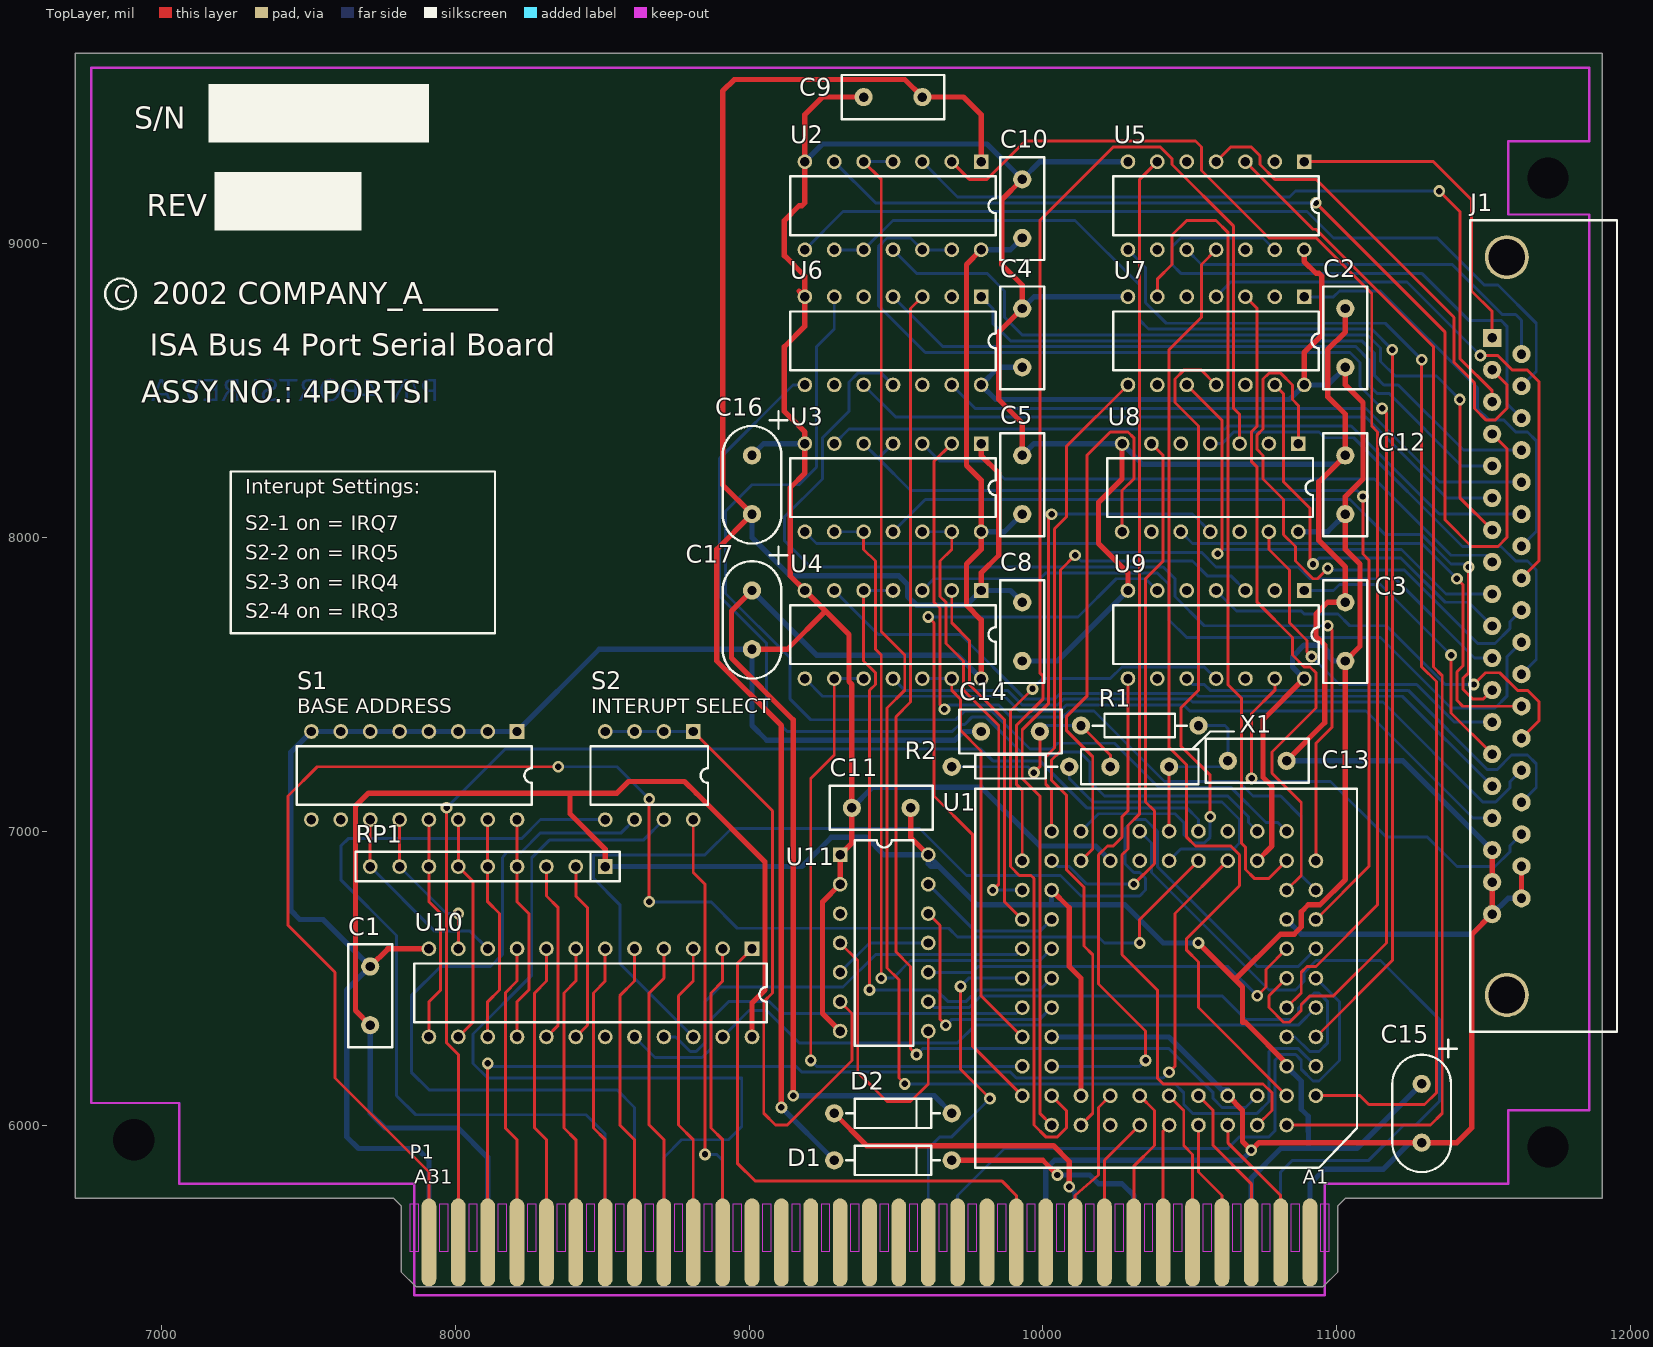
[diagram p0: TopLayer view]
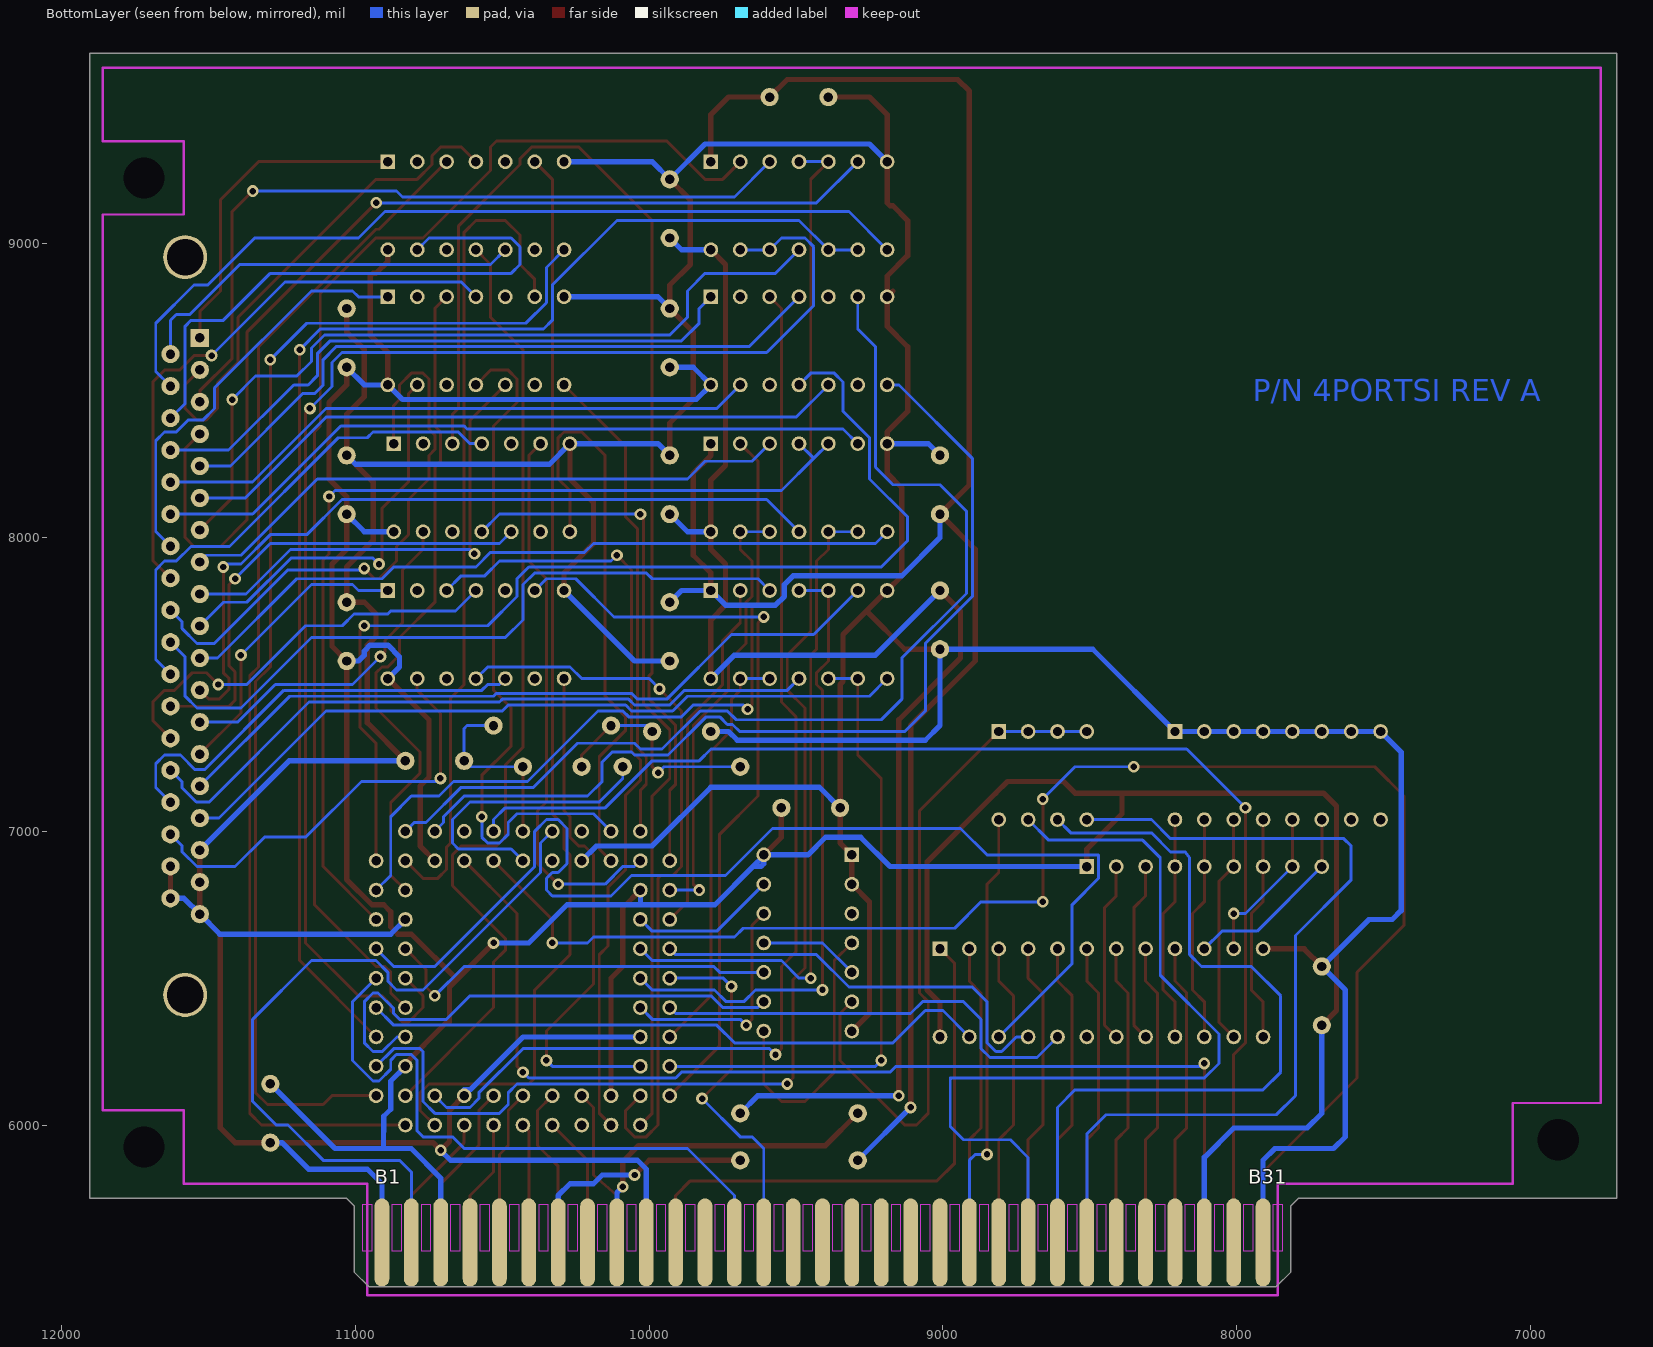
[diagram p1: BottomLayer view, seen from below]
# Altium PCB MISC95145.PcbDoc
Units mil, origin at the board's own origin, x right, y up, seen from the top; angles counter-clockwise.
Board outline 5200 x 4200 mil, 2 copper layers (TopLayer, BottomLayer); 36 components, 120 nets, 395 pads, 52 vias.

## Layer stack, top to bottom (the 12.6 mil dielectric is the usual default, probably not edited)
TopLayer: signal copper 1.4
Dielectric: core 12.6, FR-4, Dk 4.8
BottomLayer: signal copper 1.4

## Board outline
6705,9650 6705,5750 7790,5750 7815,5725 7815,5500 7865,5450 10955,5450 11005,5500 11005,5725 11030,5750 11905,5750 11905,9650

## Design rules (kind name [scope] priority, off if disabled: settings)
Clearance [All] p1: gap=10
ComponentClearance [All] p1 off: gap=10 collisioncheckmode=0
HoleSize [All] p1: absolutevalues=TRUE maxlimit=140 minlimit=1 maxpercent=80.000 minpercent=20.000
MinimumAnnularRing MinimumAnnularRing_Mtg [InPadClass('MTG')] p1: minimumring=-90
MinimumAnnularRing [All] p2: minimumring=9
PasteMaskExpansion PasteMaskExpansion_Edge [InComponent('P1')] p1: expansion=-150
PasteMaskExpansion [All] p2: expansion=0
PolygonConnect [All] p1: connectstyle=Relief reliefconductorwidth=10 reliefentries=4 polygonreliefangle="90 Angle"
RoutingLayers [All] p1: top layer=Vertical bottom layer=Horizontal
RoutingVias [All] p1: holewidth=22 width=40 viastyle="Through Hole" minholewidth=22 minwidth=40 maxholewidth=28 maxwidth=50
SolderMaskExpansion SolderMaskExpansion_Mtg [InPadClass('MTG')] p1: expansion=50
SolderMaskExpansion [All] p2: expansion=4
SupplyNets SupplyNets_1 [InNet('VCC')] p1: voltage=5.000
SupplyNets [InNet('GND')] p2: voltage=0.000
TestPointUsage [All] p1 off: valid=0 allowmultiple=FALSE
Testpoint [All] p1 off: side=15 testpointundercomponent=TRUE minsize=40 maxsize=100 preferedsize=60 minholesize=0 maxholesize=40 preferedholesize=32 testpointgrid=1 style=1023 order=1234567890
Width +12V [InNet('+12V')] p1: maxlimit=18 minlimit=18 preferedwidth=18
Width VCC [InNet('VCC')] p2: maxlimit=18 minlimit=18 preferedwidth=18
Width GND [InNet('GND')] p3: maxlimit=18 minlimit=18 preferedwidth=18
Width -12V [InNet('-12V')] p4: maxlimit=18 minlimit=18 preferedwidth=18
Width -12V_U/P [InNet('-12V_U/P')] p5: maxlimit=18 minlimit=18 preferedwidth=18
Width +12V_U/P [InNet('+12V_U/P')] p6: maxlimit=18 minlimit=18 preferedwidth=18
Width All [All] p7: maxlimit=10 minlimit=10 preferedwidth=10
14 further rules are at their usual default settings.

## Classes and differential pairs
pad class MTG: Free-1 Free-2 Free-3
net class A[0..2]: A0 A1 A2
net class D[0..7]: D0 D1 D2 D3 D4 D5 D6 D7

## Components (designator, comment, footprint, x,y, rotation, side; value= is the part's Value field where it differs from the comment)
C1 "0.1uF" RAD0.2 7710,6340 r90 top
C2 "0.1uF" RAD0.2 11030,8580 r90 top
C3 "0.1uF" RAD0.2 11030,7580 r90 top
C4 "0.1uF" RAD0.2 9930,8580 r90 top
C5 "0.1uF" RAD0.2 9930,8080 r90 top
C8 "0.1uF" RAD0.2 9930,7780 r270 top
C9 "0.1uF" RAD0.2 9590,9500 r180 top
C10 "0.1uF" RAD0.2 9930,9020 r90 top
C11 "0.1uF" RAD0.2 9550,7080 r180 top
C12 "0.1uF" RAD0.2 11030,8080 r90 top
C13 "20pF" RAD0.2 10630,7240 r0 top
C14 "50pF" RAD0.2 9990,7340 r180 top
C15 "10uF" "TANT 2M/2M" 11290,6140 r270 top
C16 "10uF" "TANT 2M/2M" 9010,8280 r270 top
C17 "10uF" "TANT 2M/2M" 9010,7820 r270 top
D1 "1N4004" DIODE0.4 9290,5880 r0 top
D2 "1N4004" DIODE0.4 9290,6040 r0 top
J1 "DB37" DB37RA/F 11530,8680 r270 top
P1 "CON AT62B" ECN-IBMXT 10910,5600 r0 top locked
R1 "1M" AXIAL0.4 10130,7360 r0 top
R2 "1K5" AXIAL0.4 10090,7220 r180 top
RP1 "10K" SIP9 8510,6880 r180 top
S1 "BASE ADDRESS" DIP16 8210,7340 r270 top
S2 "INTERUPT SELECT" DIP8 8810,7340 r270 top
U1 "TL16C554" PGA68X11_SKT 10430,6000 r270 top
U2 "1488" DIP14 9790,9280 r270 top
U3 "1488" DIP14 9790,8320 r270 top
U4 "1488" DIP14 9790,7820 r270 top
U5 "1489" DIP14 10890,9280 r270 top
U6 "1489" DIP14 9790,8820 r270 top
U7 "1489" DIP14 10890,8820 r270 top
U8 "1489" DIP14 10870,8320 r270 top
U9 "1489" DIP14 10890,7820 r270 top
U10 "P22V10" SDIP24 9010,6600 r270 top
U11 "74HC32" DIP14 9310,6920 r0 top
X1 "1.8432Mhz" XTAL1 10230,7220 r0 top

## Footprints (in the part's own frame and the unit in brackets; to place one, negate y for a bottom-side part, rotate by r counter-clockwise, add the part's x,y. Pads: shape width x height; smd on the part's side, far side on the other; paste and mask are expansions set on the pad)
AXIAL0.4 [mil]
  round 62 hole 32: 1(0,0) 2(400,0)
  silkscreen extent 40,-40 360,40
DB37RA/F [mil]
  round 150 hole 125: 0(-275,50) 0(2237,50)
  rect 62x62 hole 32: 1(0,0)
  round 62 hole 32: 2(109,0) 3(218,0) 4(327,0) 5(436,0) 6(545,0) 7(654,0) 8(763,0) 9(872,0) 10(981,0) 11(1090,0) 12(1199,0) 13(1308,0) 14(1417,0) 15(1526,0) 16(1635,0) 17(1744,0) 18(1853,0) 19(1962,0) 20(55,100) 21(164,100) 22(273,100) 23(382,100) 24(491,100) 25(600,100) 26(709,100) 27(818,100) 28(927,100) 29(1036,100) 30(1145,100) 31(1254,100) 32(1363,100) 33(1472,100) 34(1581,100) 35(1690,100) 36(1799,100) 37(1908,100)
  silkscreen extent -400,-75 2362,425
DIODE0.4 [mil]
  round 62 hole 32: A(0,0) K(400,0)
  silkscreen extent 40,-50 360,50
DIP8 [mil]
  rect 50x50 hole 32: 1(0,0)
  round 50 hole 32: 2(0,-100) 3(0,-200) 4(0,-300) 5(300,-300) 6(300,-200) 7(300,-100) 8(300,0)
  silkscreen extent 50,-350 250,50
DIP14 [mil]
  rect 50x50 hole 32: 1(0,0)
  round 50 hole 32: 2(0,-100) 3(0,-200) 4(0,-300) 5(0,-400) 6(0,-500) 7(0,-600) 8(300,-600) 9(300,-500) 10(300,-400) 11(300,-300) 12(300,-200) 13(300,-100) 14(300,0)
  silkscreen extent 50,-650 250,50
DIP16 [mil]
  rect 50x50 hole 32: 1(0,0)
  round 50 hole 32: 2(0,-100) 3(0,-200) 4(0,-300) 5(0,-400) 6(0,-500) 7(0,-600) 8(0,-700) 9(300,-700) 10(300,-600) 11(300,-500) 12(300,-400) 13(300,-300) 14(300,-200) 15(300,-100) 16(300,0)
  silkscreen extent 50,-750 250,50
ECN-IBMXT [mil]
  oval 50x300 smd: A1(0,0) A2(-100,0) A3(-200,0) A4(-300,0) A5(-400,0) A6(-500,0) A7(-600,0) A8(-700,0) A9(-800,0) A10(-900,0) A11(-1000,0) A12(-1100,0) A13(-1200,0) A14(-1300,0) A15(-1400,0) A16(-1500,0) A17(-1600,0) A18(-1700,0) A19(-1800,0) A20(-1900,0) A21(-2000,0) A22(-2100,0) A23(-2200,0) A24(-2300,0) A25(-2400,0) A26(-2500,0) A27(-2600,0) A28(-2700,0) A29(-2800,0) A30(-2900,0) A31(-3000,0)
  oval 50x300 smd far side: B1(0,0) B2(-100,0) B3(-200,0) B4(-300,0) B5(-400,0) B6(-500,0) B7(-600,0) B8(-700,0) B9(-800,0) B10(-900,0) B11(-1000,0) B12(-1100,0) B13(-1200,0) B14(-1300,0) B15(-1400,0) B16(-1500,0) B17(-1600,0) B18(-1700,0) B19(-1800,0) B20(-1900,0) B21(-2000,0) B22(-2100,0) B23(-2200,0) B24(-2300,0) B25(-2400,0) B26(-2500,0) B27(-2600,0) B28(-2700,0) B29(-2800,0) B30(-2900,0) B31(-3000,0)
PGA68X11_SKT [mil]
  round 50 hole 32: 1(0,0) 2(-100,0) 3(0,100) 4(-100,100) 5(0,200) 6(-100,200) 7(0,300) 8(-100,300) 9(0,400) 10(-100,500) 11(-100,400) 12(-200,500) 13(-200,400) 14(-300,500) 15(-300,400) 16(-400,500) 17(-400,400) 18(-500,500) 19(-500,400) 20(-600,500) 21(-600,400) 22(-700,500) 23(-700,400) 24(-800,500) 25(-800,400) 26(-900,500) 27(-1000,400) 28(-900,400) 29(-1000,300) 30(-900,300) 31(-1000,200) 32(-900,200) 33(-1000,100) 34(-900,100) 35(-1000,0) 36(-900,0) 37(-1000,-100) 38(-900,-100) 39(-1000,-200) 40(-900,-200) 41(-1000,-300) 42(-900,-300) 43(-1000,-400) 44(-900,-500) 45(-900,-400) 46(-800,-500) 47(-800,-400) 48(-700,-500) 49(-700,-400) 50(-600,-500) 51(-600,-400) 52(-500,-500) 53(-500,-400) 54(-400,-500) 55(-400,-400) 56(-300,-500) 57(-300,-400) 58(-200,-500) 59(-200,-400) 60(-100,-500) 61(0,-400) 62(-100,-400) 63(0,-300) 64(-100,-300) 65(0,-200) 66(-100,-200) 67(0,-100) 68(-100,-100)
  silkscreen extent -1145,-660 145,640
RAD0.2 [mil]
  round 62 hole 32: 1(0,0) 2(200,0)
  silkscreen extent -75,-75 275,75
SDIP24 [mil]
  rect 50x50 hole 32: 1(0,0)
  round 50 hole 32: 2(0,-100) 3(0,-200) 4(0,-300) 5(0,-400) 6(0,-500) 7(0,-600) 8(0,-700) 9(0,-800) 10(0,-900) 11(0,-1000) 12(0,-1100) 13(300,-1100) 14(300,-1000) 15(300,-900) 16(300,-800) 17(300,-700) 18(300,-600) 19(300,-500) 20(300,-400) 21(300,-300) 22(300,-200) 23(300,-100) 24(300,0)
  silkscreen extent 50,-1150 250,50
SIP9 [mil]
  rect 50x50 hole 32: 1(0,0)
  round 50 hole 32: 2(100,0) 3(200,0) 4(300,0) 5(400,0) 6(500,0) 7(600,0) 8(700,0) 9(800,0)
  silkscreen extent -50,-50 850,50
"TANT 2M/2M" [mil]
  round 62 hole 32: 1(0,0) 2(200,0)
  silkscreen extent -150,-100 300,120
XTAL1 [mil]
  round 62 hole 32: 1(0,0) 2(200,0)
  silkscreen extent -100,-60 300,60

## Free pads (board coordinates)
  round 50 hole 140: 1(6905,5950) 2(11720,5925) 3(11720,9225)

## Via types
v1: diameter 40, hole 22, TopLayer to BottomLayer, 52 vias

## Nets (pads, with @x,y where several pads share a name; then routed paths per layer and width w, separated by ;. In a path a pad name is that pad's centre, name@x,y a point inside that pad or via, vN(x,y) a via of type N, cw(c..) or ccw(c..) an arc to the next point about the centre after c; other vN are vias at no path point)
+12V: C5.1 C10.1 C17.1 D2.K U2.14 U3.14 U4.14 | length 5169.4
  TopLayer w18: C17.1 8940,7750 8940,7590 9150,7380 v1(9150,6100) ; U4.14 9790,7720 9740,7770 9740,7910 9790,7960 U3.14 9790,8196 9740,8246 9740,8930 U2.14
  BottomLayer w18: C17.1 9230,7600 9710,7600 U4.14 ; v1(9150,6100) 9630,6100 D2.K ; U3.14 9870,8020 C5.1 ; U2.14 9890,8980 C10.1
+12V_U/P: D2.A P1.B9 | length 1152.2
  TopLayer w18: D2.A 9400,5930 10036,5930 10090,5876 v1(10090,5790)
  BottomLayer w18: v1(10090,5790) 10100,5780 10110,5770 P1.B9
-12V: C8.1 C9.1 C16.2 D1.A U2.1 U3.1 U4.1 | length 6708.8
  TopLayer w18: v1(9110,6060) 9110,7360 8890,7580 8890,7960 C16.2 8910,8180 8910,9520 8950,9560 9530,9560 C9.1 9730,9500 9790,9440 U2.1 ; U4.1 9790,7880 9850,7940 9850,8220 9790,8280 U3.1
  BottomLayer w18: C16.2 9010,8000 9140,7870 9510,7870 9540,7840 9540,7800 9570,7770 9740,7770 U4.1 9890,7820 C8.1 ; v1(9110,6060) D1.A
-12V_U/P: D1.K P1.B7 | length 829.7
  TopLayer w18: D1.K 10000,5880 v1(10050,5830)
  BottomLayer w18: v1(10050,5830) 10160,5830 10190,5800 10270,5800 10310,5760 P1.B7
-CSA: U1.16 U10.23 | length 2152.5
  BottomLayer w10: U10.23 9000,6390 9060,6390 9170,6280 9710,6280 9770,6340 10870,6340 U1.16
-CSB: U1.20 U10.22 | length 3997.1
  BottomLayer w10: U10.22 8560,6550 8560,6750 8470,6840 8470,6920 8850,6920 8940,7010 9580,7010 9740,6850 10060,6850 10130,6780 10330,6780 10350,6800 10350,6840 10330,6860 10310,6860 10280,6890 10280,7010 10310,7040 10350,7040 10390,7000 10390,6880 10730,6540 10870,6540 U1.20
-CSC: U1.50 U10.21 | length 1467.7
  BottomLayer w10: U10.21 8750,6300 8800,6250 8820,6250 8850,6280 8850,6420 8900,6470 9320,6470 9430,6580 9910,6580 U1.50
-CSD: U1.54 U10.20 | length 1511.1
  BottomLayer w10: U10.20 8680,6230 8840,6230 8870,6260 8870,6360 8930,6420 9070,6420 9110,6380 9910,6380 U1.54
-RD: P1.B14 U1.52 | length 1245.4
  TopLayer w10: v1(9720,6472) 9720,6190 v1(9820,6090)
  BottomLayer w10: P1.B14 9610,5920 9650,5960 9690,5960 v1(9820,6090) ; v1(9720,6472) 9748,6500 U1.52
-WR: P1.B13 U1.18 | length 2197
  BottomLayer w10: P1.B13 9710,5760 9870,5920 10630,5920 10670,5960 10770,5960 10790,5980 10790,6220 10810,6240 10861,6240 10880,6221 10880,6190 10920,6150 10940,6150 11010,6220 11010,6420 U1.18
A0: P1.A31 U1.34 | length 5476.6
  TopLayer w10: P1.A31 7910,5840 7590,6160 7590,6520 7430,6680 7430,7120 7530,7220 v1(8350,7220) ; v1(8660,6760) v1(8660,7110) ; v1(10330,6620) 10330,6700 10370,6740 U1.34
  BottomLayer w10: v1(8350,7220) 8550,7220 v1(8660,7110) ; v1(8660,6760) 8870,6760 8960,6670 9680,6670 9710,6640 10190,6640 10210,6620 v1(10330,6620)
A1: P1.A30 U1.33 | length 4278.8
  TopLayer w10: v1(7970,7080) 7970,6280 8010,6240 P1.A30
  BottomLayer w10: v1(7970,7080) 8170,7280 9790,7280 9830,7240 9990,7240 10150,7080 10490,7080 10530,7040 U1.33
A2: P1.A29 U1.32 | length 3761.8
  TopLayer w10: P1.A29 v1(8110,6210) ; v1(10430,6180) 10450,6200 10450,6720 U1.32
  BottomLayer w10: v1(8110,6210) 8120,6200 9160,6200 9180,6180 9890,6180 9910,6160 10410,6160 v1(10430,6180)
CARD_ENABLE: U10.19
CTSA: U1.11 U5.11 | length 3331.4
  TopLayer w10: U5.11 10540,8930 10540,8750 10430,8640 10430,7286 10490,7226 10490,6980 10520,6950 10640,6950 10670,6920 10670,6815 10490,6635 10490,6595 10530,6555 10530,6400 U1.11
CTSB: U1.25 U7.3 | length 2272
  TopLayer w10: U7.3 10730,8780 10730,8380 10710,8360 10710,8260 10730,8240 10730,7780 10850,7660 10850,7600 10890,7560 10910,7560 10930,7540 10930,7420 10780,7270 10780,7198 10880,7098 10880,6850 U1.25
CTSC: U1.45 U8.6 | length 1896
  TopLayer w10: v1(10310,6820) 10380,6890 10380,7070 10350,7100 10350,7860 10410,7920 10410,8280 U8.6
  BottomLayer w10: U1.45 10050,6880 10090,6880 10150,6820 v1(10310,6820)
CTSD: U1.59 U9.8 | length 1747.7
  TopLayer w10: U9.8 10290,7070 10270,7050 10270,6980 10240,6950 10220,6950 10190,6920 10190,6480 10350,6320 v1(10350,6220)
  BottomLayer w10: U1.59 10330,6200 v1(10350,6220)
D0: P1.A9 U1.66 | length 552.9
  TopLayer w10: P1.A9 10110,5760 10190,5830 10190,6060 U1.66
D1: P1.A8 U1.67 | length 449.7
  TopLayer w10: P1.A8 10210,5880 U1.67
D2: P1.A7 U1.68 | length 549.7
  TopLayer w10: P1.A7 10310,5860 10380,5930 10380,6050 U1.68
D3: P1.A6 U1.1 | length 408.3
  TopLayer w10: P1.A6 10410,5980 U1.1
D4: P1.A5 U1.2 | length 533.1
  TopLayer w10: U1.2 10480,6050 10480,5930 10510,5900 P1.A5
D5: P1.A4 U1.3 | length 433.1
  TopLayer w10: U1.3 10530,5840 10610,5760 P1.A4
D6: P1.A3 U1.4 | length 574.6
  TopLayer w10: U1.4 10580,6050 10580,5930 10710,5800 P1.A3
D7: P1.A2 U1.5 | length 474.6
  TopLayer w10: U1.5 10630,5940 10810,5760 P1.A2
DCDA: U1.9 U5.3 | length 4069.9
  TopLayer w10: U5.3 10920,9050 10930,9050 11330,8650 11330,7560 11360,7530 11360,6040 11320,6000 U1.9
DCDB: U1.27 U6.6 | length 3625.9
  BottomLayer w10: U6.6 9290,8710 9230,8650 9230,8240 9170,8180 9010,8180 8920,8090 8920,7810 9140,7590 9140,7450 9210,7380 9704,7380 9734,7410 9826,7410 9956,7280 10030,7280 10050,7300 10244,7300 10394,7150 10640,7150 10760,7030 10800,7030 U1.27
DCDC: U1.43 U7.8 | length 1644.3
  TopLayer w10: U1.43 10030,7140 10010,7160 10010,7254 10040,7284 10040,8030 10080,8070 10080,8310 U7.8
DCDD: U1.61 U8.11 | length 2727.7
  TopLayer w10: U1.61 9990,6040 9990,7120 9930,7180 9930,7346 10020,7436 10020,8070 v1(10030,8080)
  BottomLayer w10: v1(10030,8080) 10510,8080 U8.11
DSRA: U1.10 U5.8 | length 4180.9
  TopLayer w10: U1.10 11080,6100 11110,6070 11300,6070 11340,6110 11340,7510 11290,7560 v1(11290,8606)
  BottomLayer w10: U5.8 10350,8920 10350,8800 10420,8730 11166,8730 v1(11290,8606)
DSRB: U1.26 U6.11 | length 3643.6
  TopLayer w10: U1.26 10930,7300 10984,7354 10984,7686 v1(10970,7700)
  BottomLayer w10: U6.11 9450,8560 9370,8560 9340,8530 9340,8430 9250,8340 9250,8200 9120,8070 9120,7990 9210,7900 10410,7900 10450,7860 10450,7800 10550,7700 v1(10970,7700)
DSRC: U1.44 U8.3 | length 3865.1
  TopLayer w10: U1.44 9930,7140 9910,7160 9910,7360 10000,7450 10000,7530 9990,7540 9990,9080 10240,9330 10400,9330 10440,9290 10440,9270 10650,9060 10650,8440 10670,8420 U8.3
DSRD: U1.60 U9.6 | length 2613
  TopLayer w10: v1(9610,7730) 9630,7710 9630,7120 9760,6990 9760,6270 U1.60
  BottomLayer w10: v1(9610,7730) 10120,7730 10250,7860 10350,7860 U9.6
DTRA: U1.12 U2.4 U2.5 | length 5028.1
  TopLayer w10: U2.5 9450,9220 9450,7680 9530,7600 9530,7480 9470,7420 9470,6535 9510,6495 9510,6160 v1(9530,6140)
  BottomLayer w10: U2.5 U2.4 ; v1(9530,6140) 10450,6140 10480,6110 10480,6070 10510,6040 10730,6040 10770,6080 10770,6250 10780,6260 10870,6260 U1.12
DTRB: U1.24 U3.2 | length 2608.8
  TopLayer w10: v1(9665,7416) 9650,7431 9650,7760 9630,7780 9630,8260 U3.2
  BottomLayer w10: v1(9665,7416) 9679,7430 9850,7430 9890,7390 10070,7390 10090,7410 10174,7410 10414,7170 10666,7170 10716,7120 10810,7120 10880,7050 10880,6850 U1.24
DTRC: U1.46 U3.12 U3.13 | length 1527.7
  TopLayer w10: U3.13 9690,7960 9650,7920 9650,7800 9670,7780 9670,7640 9730,7580 9730,7480 9850,7360 9850,6820 v1(9830,6800)
  BottomLayer w10: U3.12 U3.13 ; v1(9830,6800) U1.46
DTRD: U1.58 U4.9 U4.10 | length 2161.4
  TopLayer w10: v1(9210,6220) 9210,7180 9290,7260 U4.9
  BottomLayer w10: v1(9210,6220) 9230,6200 U1.58 ; U4.9 U4.10
GND: C1.2 C2.2 C3.2 C4.2 C5.2 C8.2 C9.2 C10.2 C11.2 C12.2 C13.2 C14.2 C15.2 C16.1 C17.2 J1.17 J1.18 J1.19 J1.36 J1.37 P1.B1 P1.B10 P1.B31 S1.1 S1.2 S1.3 S1.4 S1.5 S1.6 S1.7 S1.8 U1.6 U1.23 U1.40 U1.57 U2.7 U3.7 U4.7 U5.7 U6.7 U7.7 U8.7 U9.7 U10.12 U11.1 U11.2 U11.7 | length 23020
  TopLayer w18: C1.2 7770,6600 U10.12 ; C17.2 9130,7620 9260,7750 ; 9170,8840 U6.7 ; U11.7 9250,6380 9250,6760 U11.2 U11.1 9350,6960 C11.2 9350,7500 9340,7510 9340,7670 9260,7750 ; C9.2 9250,9500 9190,9440 U2.7 9190,9140 9180,9130 9170,9130 9120,9080 9120,8960 9190,8890 U6.7 ; C5.2 9930,8390 9850,8470 9850,8700 C4.2 9930,8860 9860,8930 9860,9150 C10.2 ; U8.7 10270,8200 10190,8120 10190,7980 10290,7880 U9.7 ; U1.6 10680,6050 10680,5944 v1(10710,5914) 10736,5940 C15.2 11410,5940 11460,5990 11460,6648 J1.19 J1.18 J1.17 ; C13.2 10960,7370 10960,7634 10930,7664 10930,7740 10970,7780 C3.2 11030,7900 10940,7990 10940,8190 C12.2 11030,8420 10970,8480 10970,8640 11030,8700 C2.2 ; J1.37 J1.36 ; U6.7 9190,8720 9120,8650 9120,8430 9190,8360 U3.7 9190,8220 9140,8170 9140,7870 U4.7 9260,7750
  BottomLayer w18: P1.B31 7910,5880 7870,5920 7670,5920 7630,5960 7630,6460 C1.2 7550,6700 7470,6700 7440,6730 7440,7270 S1.8 S1.7 S1.6 S1.5 S1.4 S1.3 S1.2 S1.1 8490,7620 C17.2 9010,7360 9060,7310 9700,7310 9730,7340 C14.2 ; C16.1 9050,8320 U3.7 ; U2.7 9250,9340 9810,9340 C10.2 9990,9280 U5.7 ; C11.2 9420,7150 9790,7150 9990,6950 10180,6950 U1.40 ; C8.2 10050,7580 U9.7 ; C5.2 9970,8320 U8.7 10340,8250 11000,8250 C12.2 ; C4.2 9970,8820 U7.7 ; P1.B10 10010,5850 10040,5880 10676,5880 v1(10710,5914) ; U1.57 10430,6300 10610,6120 10630,6120 U1.6 ; U1.23 10880,6650 11462,6650 J1.19 11584,6772 J1.37 ; C13.2 11226,7240 J1.17 ; P1.B1 10910,5800 10960,5850 11160,5850 11250,5940 C15.2
INTA: U1.15 U11.9 | length 1790.8
  BottomLayer w10: U11.9 9630,6400 9750,6400 9790,6440 10610,6440 10690,6360 10850,6360 10870,6380 10870,6397 10923,6450 10940,6450 10970,6420 10970,6280 10940,6250 10909,6250 10859,6300 U1.15
INTB: U1.21 U11.10 | length 1371.1
  TopLayer w10: v1(10730,6440) 10760,6470 10760,6530 U1.21
  BottomLayer w10: U11.10 9760,6520 9780,6540 10630,6540 v1(10730,6440)
INTC: U1.49 U11.13 | length 502.8
  BottomLayer w10: U11.13 9770,6660 9990,6660 U1.49
INTD: U1.55 U11.12 | length 789.7
  TopLayer w10: U11.12 9650,6680 9650,6360 v1(9670,6340)
  BottomLayer w10: v1(9670,6340) 9690,6360 9990,6360 U1.55
J1: J1.1 U5.1 | length 1122.8
  TopLayer w10: U5.1 11330,9280 11460,9150 11460,8840 11530,8770 J1.1
J2: J1.20 U5.10 | length 1354.4
  BottomLayer w10: U5.10 10540,8930 11394,8930 11564,8760 11610,8760 11630,8740 J1.20
J3: J1.2 U5.4 | length 1722.4
  TopLayer w10: U5.4 10640,9330 10710,9330 10740,9300 10740,9270 10790,9220 10930,9220 11400,8750 11400,8597 11470,8527 11470,8440 11510,8400 11540,8400 11580,8440 11580,8521 J1.2
J4: J1.21 U2.8 | length 2936
  BottomLayer w10: U2.8 9320,9110 10900,9110 10990,9020 11343,9020 11503,8860 11550,8860 11680,8730 11680,8566 J1.21
J5: J1.3 U2.3 | length 2610.5
  TopLayer w10: v1(11350,9180) 11420,9110 11420,8610 11530,8500 J1.3
  BottomLayer w10: U2.3 9710,9160 10840,9160 10860,9180 v1(11350,9180)
J6: J1.22 U5.13 | length 1999.7
  BottomLayer w10: U5.13 10750,9020 10470,9020 10440,8990 10440,8930 10470,8900 11290,8900 11450,8740 11560,8740 11580,8720 11580,8457 J1.22
J7: J1.4 U2.6 | length 3593.1
  TopLayer w10: v1(10929,9140) 11370,8699 11370,8060 11460,7970 11550,7970 11580,8000 11580,8303 J1.4
  BottomLayer w10: U2.6 9430,9140 v1(10929,9140)
J8: J1.23 U6.1 | length 2129.4
  BottomLayer w10: U6.1 9830,8780 9830,8730 9890,8670 11086,8670 11130,8626 11130,8551 11161,8520 11210,8520 11432,8298 J1.23
J11: J1.5 U6.4 | length 2329
  BottomLayer w10: U6.4 9660,8650 11066,8650 11110,8606 11110,8520 11140,8490 11180,8490 11426,8244 J1.5
J12: J1.24 U6.13 | length 2077.1
  BottomLayer w10: U6.13 9770,8440 11100,8440 11351,8189 J1.24
J13: J1.6 U6.10 | length 2299.5
  BottomLayer w10: U6.10 9500,8410 11100,8410 11375,8135 J1.6
J14: J1.25 U3.6 | length 2489.1
  BottomLayer w10: U3.6 9340,8370 10620,8370 10630,8380 11050,8380 11350,8080 J1.25
J15: J1.7 U2.11 | length 2710.5
  TopLayer w10: v1(11420,8470) 11420,8136 J1.7
  BottomLayer w10: U2.11 9570,8900 9810,8900 9870,8840 9870,8750 9930,8690 11106,8690 11150,8646 11150,8600 11200,8550 11340,8550 v1(11420,8470)
J16: J1.26 U7.1 | length 1430.2
  BottomLayer w10: U7.1 10990,8820 11010,8840 11150,8840 11480,8510 11480,8440 11520,8400 11570,8400 11610,8360 11650,8360 11680,8330 11680,8021 J1.26
J17: J1.8 U3.3 | length 2106.9
  BottomLayer w10: U3.3 9650,8260 9810,8260 9870,8200 11130,8200 11390,7940 11507,7940 J1.8
J18: J1.27 U7.4 | length 1954.4
  TopLayer w10: v1(11490,8620) 11549,8620 11599,8570 11650,8570 11690,8530 11690,7922 J1.27
  BottomLayer w10: U7.4 10640,8870 11240,8870 v1(11490,8620)
J21: J1.9 U7.10 | length 1635.1
  TopLayer w10: U7.10 10610,8400 10610,7960 v1(10595,7945)
  BottomLayer w10: v1(10595,7945) 10610,7960 11221,7960 11373,7808 J1.9
J22: J1.28 U8.1 | length 1990.5
  TopLayer w10: U8.1 10870,8450 10850,8470 10850,8520 10810,8560 10770,8560 10750,8540 10750,8370 10730,8350 10730,8300 10750,8280 10750,8200 10820,8130 10820,8010 10860,7970 10860,7920 10920,7860 10935,7860 v1(10970,7895)
  BottomLayer w10: v1(10970,7895) 10975,7890 11231,7890 11481,7640 11540,7640 11590,7690 11590,7713 J1.28
J23: J1.10 U7.13 | length 1377.8
  TopLayer w10: U7.13 10820,8490 10820,8190 10910,8100 10910,7920 v1(10920,7910)
  BottomLayer w10: v1(10920,7910) 10940,7930 11220,7930 11370,7780 11449,7780 J1.10
J24: J1.29 U4.3 | length 2497
  BottomLayer w10: U4.3 9630,7860 9990,7860 10010,7880 10390,7880 10430,7840 10430,7720 10490,7660 11150,7660 11390,7420 11540,7420 11580,7460 11580,7594 J1.29
J25: J1.11 U3.8 | length 2518.1
  BottomLayer w10: U3.8 9230,7980 10190,7980 10220,7950 10540,7950 10590,7900 10870,7900 10910,7860 11200,7860 11470,7590 J1.11
J26: J1.30 U8.4 | length 1697
  BottomLayer w10: U8.4 10610,8320 10650,8360 10940,8360 10960,8340 11059,8340 11429,7970 11560,7970 11610,7920 11650,7920 11680,7890 11680,7585 J1.30
J27: J1.12 U3.11 | length 2651.5
  TopLayer w10: v1(11450,7900) 11450,7540 11430,7520 11430,7485 11465,7450 11499,7450 J1.12
  BottomLayer w10: U3.11 9600,8130 11046,8130 11166,8010 11290,8010 11390,7910 11440,7910 v1(11450,7900)
J28: J1.31 U8.10 | length 1665.1
  TopLayer w10: v1(11410,7860) 11430,7840 11430,7563 11410,7543 11410,7446 11430,7426 J1.31
  BottomLayer w10: U8.10 10510,7980 11290,7980 v1(11410,7860)
J31: J1.13 U8.13 | length 1192.4
  TopLayer w10: U8.13 10770,7960 10840,7890 10840,7710 10900,7650 10900,7610 v1(10915,7595)
  BottomLayer w10: v1(10915,7595) 11010,7500 11273,7500 11401,7372 J1.13
J32: J1.32 U9.4 | length 1438.4
  TopLayer w10: v1(11467,7500) 11507,7540 11556,7540 11616,7480 11650,7480 11690,7440 11690,7377 J1.32
  BottomLayer w10: U9.4 10660,7750 10880,7750 10890,7740 11005,7740 11045,7700 11170,7700 11370,7500 v1(11467,7500)
J33: J1.14 U9.1 | length 1002.7
  TopLayer w10: v1(11390,7600) 11390,7403 J1.14
  BottomLayer w10: U9.1 10990,7820 11010,7840 11150,7840 v1(11390,7600)
J34: J1.33 U4.11 | length 2387
  BottomLayer w10: U4.11 9530,7480 9880,7480 9930,7430 10050,7430 10070,7450 10500,7450 10510,7440 11158,7440 11498,7100 11542,7100 11590,7148 11590,7168 J1.33
J35: J1.15 U4.6 | length 2532.4
  BottomLayer w10: U4.6 9440,7670 9720,7670 9940,7450 10040,7450 10060,7470 10520,7470 10530,7460 11224,7460 J1.15
J36: J1.34 U9.10 | length 1503.3
  BottomLayer w10: U9.10 10510,7500 10550,7500 10570,7480 11244,7480 11514,7210 11546,7210 11596,7260 11650,7260 11680,7230 11680,7149 J1.34
J37: J1.16 U4.8 | length 2553.3
  BottomLayer w10: U4.8 9250,7460 9870,7460 9920,7410 10060,7410 10080,7430 10480,7430 10500,7410 11100,7410 11465,7045 J1.16
J38: J1.35 U9.13 | length 1473.3
  TopLayer w10: v1(10711,7180) 10711,7401 10790,7480 U9.13
  BottomLayer w10: v1(10711,7180) 10721,7170 10980,7170 11170,6980 11310,6980 11410,6880 11540,6880 11590,6930 11590,6950 J1.35
NetC13_1: C13.1 R1.2 U1.35 X1.2 | length 642.4
  TopLayer w10: U1.35 X1.2
  BottomLayer w10: X1.2 10610,7220 C13.1 10630,7350 10620,7360 R1.2
NetC14_1: C14.1 R1.1 R2.2 X1.1 | length 766.3
  TopLayer w10: v1(9970,7200) 9990,7220 C14.1 ; R1.1 10230,7260 X1.1
  BottomLayer w10: R2.2 9950,7220 v1(9970,7200) ; C14.1 10010,7360 R1.1
NetP1_A11: P1.A11 U10.1 | length 1906.3
  TopLayer w10: U10.1 8960,6550 8960,5870 9020,5810 9860,5810 9910,5760 P1.A11
NetP1_A21: P1.A21 U10.2 | length 1033.1
  TopLayer w10: P1.A21 8910,5950 8870,5990 8870,6450 8910,6490 U10.2
NetP1_A22: P1.A22 U10.3 | length 1041.4
  TopLayer w10: P1.A22 8810,5950 8760,6000 8760,6440 8810,6490 U10.3
NetP1_A23: P1.A23 U10.4 | length 1041.4
  TopLayer w10: P1.A23 8710,5950 8660,6000 8660,6450 8710,6500 U10.4
NetP1_A24: P1.A24 U10.5 | length 1041.4
  TopLayer w10: P1.A24 8610,5950 8560,6000 8560,6440 8610,6490 U10.5
NetP1_A25: P1.A25 U10.6 | length 1033.1
  TopLayer w10: P1.A25 8510,5950 8470,5990 8470,6450 8510,6490 U10.6
NetP1_A26: P1.A26 U10.7 | length 1033.1
  TopLayer w10: P1.A26 8410,5950 8370,5990 8370,6450 8410,6490 U10.7
NetP1_A27: P1.A27 U10.8 | length 1033.1
  TopLayer w10: P1.A27 8310,5950 8270,5990 8270,6450 8310,6490 U10.8
NetP1_A28: P1.A28 U10.9 | length 1033.1
  TopLayer w10: P1.A28 8210,5950 8170,5990 8170,6450 8210,6490 U10.9
NetP1_B21: P1.B21 S2.8 | length 1504.9
  TopLayer w10: S2.8 8810,6860 8850,6820 v1(8850,5900)
  BottomLayer w10: v1(8850,5900) 8890,5900 8910,5880 P1.B21
NetP1_B23: P1.B23 S2.7 | length 2993
  BottomLayer w10: P1.B23 8710,5890 8770,5950 8930,5950 8975,5995 8975,6155 ; S2.7 8640,6970 8320,6970 8260,6910 8260,6510 8060,6310 8060,6210 8110,6160 8970,6160 ; 8970,6160 8975,6155 ; 8970,6160 8975,6160 8975,6155
NetP1_B24: P1.B24 S2.6 | length 2733.3
  BottomLayer w10: P1.B24 8610,6060 8550,6120 7910,6120 7850,6180 7850,6440 7950,6540 8120,6540 8160,6580 8160,6910 8175,6930 8225,6930 8290,6995 8565,6995 S2.6
NetP1_B25: P1.B25 S2.5 | length 3014.8
  BottomLayer w10: P1.B25@8510,5585 8510,5970 8445,6035 7865,6035 7800,6100 7800,6645 7610,6835 7610,6950 7635,6975 8225,6975 8290,7040 S2.5
NetR2_1: R2.1 U1.36 | length 1022.8
  BottomLayer w10: R2.1 10090,7180 10170,7100 10610,7100 10670,7040 10670,6960 10650,6940 10470,6940 U1.36
NetRP1_2: RP1.2 U10.18 | length 613.1
  TopLayer w10: U10.18 8450,6340 8450,6740 8410,6780 RP1.2
NetRP1_3: RP1.3 U10.17 | length 613.1
  TopLayer w10: U10.17 8350,6340 8350,6740 8310,6780 RP1.3
NetRP1_4: RP1.4 S1.16 U10.16 | length 773.1
  TopLayer w10: U10.16 8210,6420 8250,6460 8250,6720 8210,6760 RP1.4 S1.16
NetRP1_5: RP1.5 S1.15 U10.15 | length 773.1
  TopLayer w10: U10.15 8110,6420 8150,6460 8150,6720 8110,6760 RP1.5 S1.15
NetRP1_6: RP1.6 S1.14 U10.14 | length 781.4
  TopLayer w10: U10.14 8060,6350 8060,6830 RP1.6 S1.14
NetRP1_7: RP1.7 S1.13 U10.13 | length 773.1
  TopLayer w10: U10.13 7910,6420 7950,6460 7950,6720 7910,6760 RP1.7 S1.13
NetRP1_8: RP1.8 S1.12 U10.11 | length 546.3
  TopLayer w10: RP1.8 S1.12 ; U10.11 v1(8010,6720)
  BottomLayer w10: RP1.8 7970,6720 v1(8010,6720)
NetRP1_9: RP1.9 S1.11 U10.10 | length 676
  TopLayer w10: RP1.9 S1.11
  BottomLayer w10: RP1.9 7930,6660 8050,6660 U10.10
NetS2_1: S2.1 S2.2 S2.3 S2.4 U11.6 | length 2348.5
  TopLayer w10: S2.1 9080,7070 9080,6450 9050,6420 9050,6040 9090,6000 9130,6000 9350,6220 9350,6380 U11.6
  BottomLayer w10: S2.4 S2.3 S2.2 S2.1
NetU11_4: U11.4 U11.8 | length 951.1
  TopLayer w10: U11.4 9370,6560 9370,6180 9470,6080 9550,6080 9610,6140 U11.8
NetU11_5: U11.5 U11.11 | length 341.4
  BottomLayer w10: U11.5 9410,6620 U11.11
RESET: P1.B2 U1.37 | length 2603.5
  BottomLayer w10: U1.37 10370,6960 10370,6860 10770,6460 10860,6460 10890,6490 10890,6520 10930,6560 11150,6560 11350,6360 11350,6080 11270,6000 11230,6000 11110,5880 10850,5880 10810,5840 P1.B2
RIA: U1.8 U6.3 | length 3925.7
  TopLayer w10: v1(9570,6240) 9550,6260 9550,6540 9500,6590 9500,7390 9550,7440 9550,8780 U6.3
  BottomLayer w10: v1(9570,6240) 9590,6260 10430,6260 10580,6110 10580,6090 10610,6060 10690,6060 U1.8
RIB: U1.28 U7.6 | length 2830.1
  TopLayer w10: U7.6 10390,8880 10440,8930 10440,9030 10490,9080 10590,9080 10630,9040 10630,7500 10676,7454 10676,6960 10690,6946 10690,6870 10720,6840 10770,6840 U1.28
RIC: U1.42 U8.8 | length 2000.8
  TopLayer w10: U1.42 10170,6940 10170,7254 10080,7344 10080,7390 10150,7460 10150,8280 10230,8360 10290,8360 10310,8340 10310,8200 10270,8160 U8.8
RID: U1.62 U9.11 | length 2515
  TopLayer w10: v1(9965,7485) 9890,7410 9890,6880 9920,6850 9960,6850 9970,6840 9970,6000 10010,5960 10050,5960 10080,5990 10080,6050 U1.62
  BottomLayer w10: v1(9965,7485) 10000,7520 10230,7520 10270,7560 10550,7560 U9.11
RTSA: U1.14 U2.9 U2.10 | length 4641.7
  TopLayer w10: U1.14 11190,6560 v1(11190,8640)
  BottomLayer w10: U2.9 U2.10 9490,9080 10110,9080 10330,8860 10330,8740 10360,8710 11120,8710 v1(11190,8640)
RTSB: U1.22 U3.4 U3.5 | length 3438.8
  TopLayer w10: U1.22 11110,6880 11110,7924 11090,7944 v1(11090,8140)
  BottomLayer w10: U3.4 9440,8270 ; v1(11090,8140) 11070,8160 9550,8160 9440,8270 ; 9440,8270 U3.5 9440,8270
RTSC: U1.48 U4.2 | length 1219.4
  TopLayer w10: U4.2 9690,7710 9750,7650 9750,7500 9870,7380 9870,6760 U1.48
RTSD: U1.56 U4.12 U4.13 | length 1419.4
  TopLayer w10: U4.13 9690,7480 9720,7450 9720,7344 9790,7274 9790,6440 U1.56
  BottomLayer w10: U4.12 U4.13
RXA: U1.7 U5.6 | length 3760.8
  TopLayer w10: U5.6 10330,9220 10330,7060 10290,7020 10290,6940 10270,6920 10270,6580 10390,6460 10390,6160 10410,6140 10750,6140 10780,6110 10780,6050 U1.7
RXB: U1.29 U6.8 | length 3259.7
  BottomLayer w10: U6.8 9150,8520 8900,8270 8900,7800 9060,7640 9060,7410 9130,7340 9692,7340 9716,7364 9734,7364 9760,7390 9806,7390 9936,7260 10050,7260 10060,7270 10126,7270 10160,7236 10160,7170 10210,7120 10630,7120 10700,7050 10700,7030 U1.29
RXC: U1.41 U7.11 | length 2370.5
  TopLayer w10: v1(10570,7050) 10570,7191 10470,7291 10470,7420 10530,7480 10530,8380 10450,8460 10450,8540 10480,8570 10540,8570 U7.11
  BottomLayer w10: U1.41 10190,7060 10450,7060 10480,7030 10480,6990 10510,6960 10550,6960 10570,6980 v1(10570,7050)
RXD: U1.63 U9.3 | length 2677.4
  TopLayer w10: v1(10110,7940) 10060,7890 10060,7273 10030,7243 10030,7174 10080,7124 10080,6870 10140,6810 10140,6610 10170,6580 10170,6040 U1.63
  BottomLayer w10: v1(10110,7940) 10130,7920 10510,7920 10560,7870 10640,7870 U9.3
TXA: U1.17 U2.2 | length 4355.8
  TopLayer w10: U2.2 9750,9220 9810,9220 9940,9350 10520,9350 10540,9330 10540,9250 10770,9020 10931,9020 11120,8831 11120,8380 11140,8360 11140,6750 10930,6540 10900,6540 10880,6520 10880,6450 U1.17
TXB: U1.19 U2.12 U2.13 | length 4881.7
  TopLayer w10: U1.19 10770,6440 10770,6400 10820,6350 10840,6350 10880,6390 10880,6410 10910,6440 10990,6440 11170,6620 11170,8425 v1(11155,8440)
  BottomLayer w10: U2.13 U2.12 9550,9020 9470,9020 9440,8990 9440,8790 9600,8630 11046,8630 11080,8596 11080,8515 v1(11155,8440)
TXC: U1.51 U3.9 U3.10 | length 2266.3
  TopLayer w10: U3.10 9390,7960 9430,7920 9430,7620 9450,7600 v1(9450,6500)
  BottomLayer w10: U3.9 U3.10 ; v1(9450,6500) 9490,6500 9550,6560 9990,6560 U1.51
TXD: U1.53 U4.4 U4.5 | length 2154.6
  TopLayer w10: U4.5 9390,7580 9430,7540 9430,7500 9410,7480 v1(9410,6460)
  BottomLayer w10: U4.5 U4.4 ; v1(9410,6460) 9638,6460 9678,6420 9738,6420 9778,6460 9990,6460 U1.53
VCC: C1.1 C2.1 C3.1 C4.1 C11.1 C12.1 C15.1 P1.B3 P1.B29 RP1.1 U1.13 U1.30 U1.47 U1.64 U5.14 U6.14 U7.14 U8.14 U9.14 U10.24 U11.14 | length 14961.1
  TopLayer w18: C1.1 7660,6390 7660,7086 7704,7130 8390,7130 ; RP1.1 8510,6940 8390,7060 8390,7130 ; U10.24 9010,6416 9054,6460 9054,6896 8820,7130 8780,7170 8590,7170 8550,7130 8390,7130 ; C11.1 9550,6980 U11.14 ; U1.47 10090,6740 10090,6540 10130,6500 U1.64 ; v1(10530,6620) 10655,6495 ; U1.30 10780,6950 10780,7154 10750,7184 10750,7380 U9.14 ; U1.13 10840,6200 10690,6350 10680,6350 10680,6470 ; U7.14 10890,8630 10950,8690 10950,8890 10940,8900 10930,8900 10890,8940 U5.14 ; C2.1 11030,8520 11090,8460 11090,8200 11030,8140 C12.1 11030,7960 11080,7910 11080,7630 C3.1 11030,6836 10944,6750 10904,6750 10880,6726 10880,6674 10856,6650 10810,6650 10655,6495 ; 10655,6495 10680,6470 ; 10655,6495 10680,6470
  BottomLayer w18: C1.1 7710,6040 7760,5990 8010,5990 8110,5890 P1.B29 ; RP1.1 9180,6880 9280,6980 9400,6980 9460,6920 U11.14@9606,6920 ; C4.1 9850,8580 U6.14 9840,8470 10840,8470 U7.14 10970,8520 C2.1 ; U1.47 10030,6750 ; v1(10530,6620) 10410,6620 10280,6750 10030,6750 ; P1.B3 10710,5820 10810,5920 10905,5920 ; U1.13 10880,6150 10880,6054 10904,6030 10905,5920 ; U8.14 10970,8020 C12.1 ; U9.14 10850,7560 10850,7594 10890,7634 10950,7634 10970,7614 10970,7600 10990,7580 C3.1 ; C15.1 11070,5920 10905,5920 ; U11.14@9606,6920 U11.14@9610,6916 ; U11.14@9606,6920 U11.14 U11.14@9610,6916 ; U11.14@9610,6916 9646,6880 ; U11.14@9610,6916 9610,6890 9620,6880 9646,6880 ; 9646,6880 9776,6750 10030,6750
pads on no net: J1.0 P1.A1 P1.A10 P1.A12 P1.A13 P1.A14 P1.A15 P1.A16 P1.A17 P1.A18 P1.A19 P1.A20 P1.B4 P1.B5 P1.B6 P1.B8 P1.B11 P1.B12 P1.B15 P1.B16 P1.B17 P1.B18 P1.B19 P1.B20 P1.B22 P1.B26 P1.B27 P1.B28 P1.B30 S1.9 S1.10 U1.31 U1.38 U1.39 U1.65 U5.2 U5.5 U5.9 U5.12 U6.2 U6.5 U6.9 U6.12 U7.2 U7.5 U7.9 U7.12 U8.2 U8.5 U8.9 U8.12 U9.2 U9.5 U9.9 U9.12 U11.3

## Keep-outs
KeepOutLayer:
  rectangle: 10845,5570 10875,5730
  rectangle: 10945,5570 10975,5730
  rectangle: 10745,5570 10775,5730
  rectangle: 10645,5570 10675,5730
  rectangle: 10545,5570 10575,5730
  rectangle: 10445,5570 10475,5730
  rectangle: 10345,5570 10375,5730
  rectangle: 10245,5570 10275,5730
  rectangle: 10145,5570 10175,5730
  rectangle: 10045,5570 10075,5730
  rectangle: 9945,5570 9975,5730
  rectangle: 9845,5570 9875,5730
  rectangle: 9745,5570 9775,5730
  rectangle: 9645,5570 9675,5730
  rectangle: 9545,5570 9575,5730
  rectangle: 9445,5570 9475,5730
  rectangle: 9345,5570 9375,5730
  rectangle: 9245,5570 9275,5730
  rectangle: 9145,5570 9175,5730
  rectangle: 9045,5570 9075,5730
  rectangle: 8945,5570 8975,5730
  rectangle: 8845,5570 8875,5730
  rectangle: 8745,5570 8775,5730
  rectangle: 8645,5570 8675,5730
  rectangle: 8545,5570 8575,5730
  rectangle: 8445,5570 8475,5730
  rectangle: 8345,5570 8375,5730
  rectangle: 8245,5570 8275,5730
  rectangle: 8145,5570 8175,5730
  rectangle: 8045,5570 8075,5730
  rectangle: 7945,5570 7975,5730
  rectangle: 7845,5570 7875,5730
  lines w8: 6760,6075 7060,6075 7060,5800 7860,5800 7860,5420 10960,5420 10960,5800 11585,5800 11585,6050 11860,6050 11860,9100 11585,9100 11585,9350 11860,9350 11860,9600 6760,9600 6760,6075

## Other copper
TopLayer:
  text ".GTL" at 13870,7205 h90
BottomLayer:
  text "P/N 4PORTSI REV A" at 7945,8465 h75
  text ".GBL" at 13870,7205 h90

## Silkscreen, mask and mechanical layers (free items; w line width, h text height)
TopOverlay:
  circle w8: c6860,8830 r52.2
  rectangle: 7160,9345 7910,9545
  rectangle: 7180,9045 7680,9245
  lines w8: 10510,7280 10570,7340 10650,7340 ; 7235,7675 8135,7675 8135,8225 7235,8225 7235,7675
  text "S/N" at 6907.5,9392.5 h75
  text "REV" at 6950,9095 h75
  text "C" at 6837,8800.5 h60
  text "2002 COMPANY_A_____" at 6967.5,8795 h75
  text "ISA Bus 4 Port Serial Board" at 6960,8620 h75
  text "ASSY NO.: 4PORTSI" at 6930,8460 h75
  text "Interupt Settings:" at 7285,8150 h50
  text "S2-1 on = IRQ7" at 7285,8025 h50
  text "S2-2 on = IRQ5" at 7285,7925 h50
  text "S2-3 on = IRQ4" at 7285,7825 h50
  text "S2-4 on = IRQ3" at 7285,7725 h50
  text ".GTO" at 13870,7205 h90
TopPaste:
  text ".GTP" at 16660,3945 h90
  text ".GTP" at 15075,3595 h90
BottomPaste:
  text ".GBP" at 16660,3945 h90
  text ".GBP" at 15075,3595 h90
TopSolder:
  rectangle: 7785,5380 11035,5755
  text ".GTS" at 16660,3945 h90
  text ".GTS" at 15075,3595 h90
BottomSolder:
  rectangle: 7785,5380 11035,5755
  text ".GBS" at 16660,3945 h90
  text ".GBS" at 15075,3595 h90
Mechanical1:
  the board outline again, w10
Mechanical3:
  lines w10: 11595,5875 11595,5825 11645,5825 ; 11595,5900 11595,5950 ; 11595,5975 11595,6025 11645,6025 ; 11595,9175 11595,9125 11645,9125 ; 11595,9200 11595,9250 ; 11595,9275 11595,9325 11645,9325 ; 11670,5825 11720,5825 ; 11670,6025 11720,6025 ; 11670,9125 11720,9125 ; 11670,9325 11720,9325 ; 11745,5825 11795,5825 ; 11745,6025 11795,6025 ; 11745,9125 11795,9125 ; 11745,9325 11795,9325 ; 11820,5825 11870,5825 ; 11820,6025 11870,6025 ; 11820,9125 11870,9125 ; 11820,9325 11870,9325 ; 11905,5825 11945,5825 11945,5090 11970,5090 11970,9400 12395,9400 12395,9425 11945,9425 11945,9325 11905,9325 ; 11905,6025 11945,6025 11945,9125 11905,9125
Mechanical4:
  circle w10: c7825,5470 r100
  lines w10: 12575,6735 12650,6660 12725,6735 12800,6660 12875,6735 12950,6660 13025,6735 ; 13056.25,5653.75 13300,5410 13500,5410 ; 14715,6700 15440,6700 ; 15445,5330 15195,5330 15488.75,5623.75 ; 16395,5530 16395,5930 16595,6030 16195,6130 16395,6230 16395,6630 ; 7683.67,5416.32 7683.67,5471.32 7703.67,5421.32 7683.67,5416.32 ; 7683.87,5471.16 7685,5525 7705.36,5521.79 7683.87,5471.16 ; 12950,5760 13075,5672.5 13037.5,5635 12950,5760 ; 15470,5642.5 15595,5730 15507.5,5605 15470,5642.5
  lines w20: 12600,6710 12600,5810 12700,5710 12900,5710 13000,5810 13000,6710 ; 15495,6630 15495,5830 15695,5630 16395,5630
  text ".LAYER_NAME" at 12760,7199.99 h90
  text "DETAIL A" at 13770,6165 h120
  text "SEE" at 7285,5525 h75
  text "o" at 14225,5435 h60
  text "DETAIL A" at 7160,5375 h75
  text ".020 X 45  CHAMFER" at 13575,5360 h90
  text "o" at 16170,5355 h60
  text "0.05 X 45  CHAMFER" at 15520,5280 h90
  text "BOTH SIDES" at 13575,5185 h90
  text "TYP 4 PLCS" at 15520,5105 h90
  text "ENTIRE LENGTH OF" at 13575,5010 h90
  text "EDGE CONNECTOR" at 13575,4835 h90
  text "4 Port Serial Interface" at 14180,4015 h130
Mechanical16:
  drawing of 1874 lines, arcs and shapes, not listed
  text "1" at 7127,10465 h70
  text "2" at 9987,10465 h70
  text "3" at 12867,10465 h70
  text "4" at 15737,10465 h70
  text "A" at 5775,9559 h70
  text "A" at 17075,9559 h70
  text "B" at 5775,7667 h70
  text "B" at 17075,7667 h70
  text "C" at 5775,5757 h70
  text "C" at 17075,5757 h70
  text "ENGINEER:" at 12550,4300 h45
  text "TITLE:" at 14050,4300 h45
  text "PCB DESIGNER:" at 12550,4005 h45
  text "D" at 5775,3867 h70
  text "D" at 17075,3867 h70
  text "DATE:" at 12550,3700 h45
  text "PART NO.:" at 14050,3700 h45
  text "REV:" at 16150,3700 h45
  text "COMPANY_A_____" at 11250,3600 h70
  text ".PRINT_DATE" at 12600,3580 h70
  text "xxxxxxxxxxxxxxxxx" at 11250,3500 h70
  text "xxxxxxxxxxxxxx" at 11250,3400 h70
  text "FILE NAME:" at 12550,3400 h45
  text "DWG NO:" at 14050,3400 h45
  text "SCALE:" at 16150,3400 h45
  text "xxxxxxxx" at 11250,3300 h70
  text ".PCB_FILE_NAME_NO_PATH" at 12600,3280 h70
  text "1" at 7127,3065 h70
  text "2" at 9987,3065 h70
  text "3" at 12867,3065 h70
  text "4" at 15737,3065 h70
DrillDrawing:
  text ".LEGEND" at 12780,7600 h90
  text "Drilling Details." at 12780,7400 h90

## Dimensions
6905,5950 to 6705,5750 on Mechanical4
6905,5950 to 6705,5750 on Mechanical4